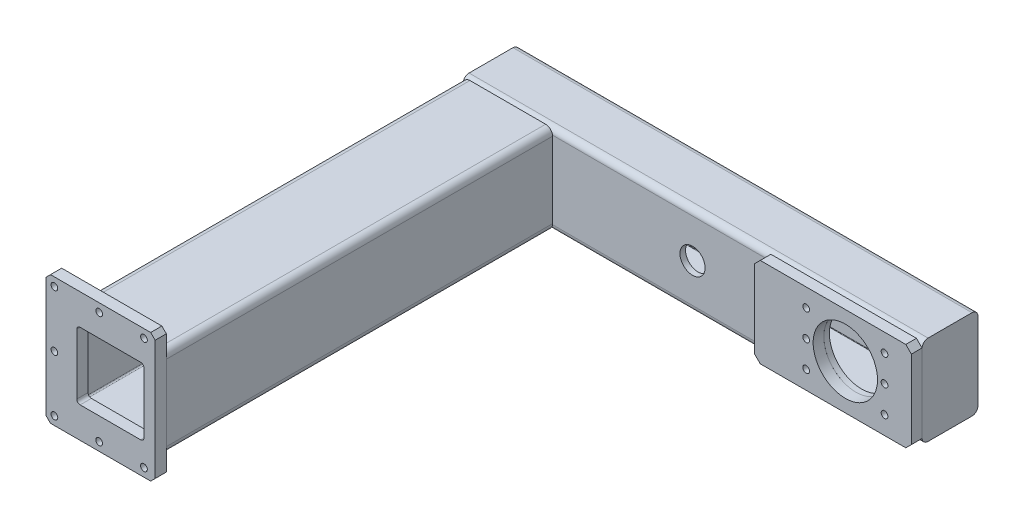
SolidWorks part; units mm, degrees
ref_plane "Front Plane" through (0, 0, 0) normal (0, 0, 1) x (1, 0, 0)
ref_plane "Top Plane" through (0, 0, 0) normal (0, 1, 0) x (1, 0, 0)
ref_plane "Right Plane" through (0, 0, 0) normal (1, 0, 0) x (0, 0, -1)
sketch "Sketch3" plane through (0, 0, 0) normal (0, 1, 0) x (1, 0, 0)
  line L0 (0, 0) -> (0, -740)
  line L1 (0, 0) -> (740, 0)
  dimension "D1" = 740
  dimension "D2" = 740
other "Structural Member1"
ref_plane "Plane1" through (0, 0, 0) normal (0, 0, 1) x (1, 0, 0)
sketch "Sketch1" plane through (0, 0, 0) normal (0, 0, 1) x (1, 0, 0)
  line L0 (-67.6073, -70) -> (67.6073, -70)
  line L1 (-70, -67.6073) -> (-70, 67.6073)
  line L2 (67.6073, 70) -> (-67.6073, 70)
  line L3 (70, 67.6073) -> (70, -67.6073)
  line L4 (-67.6073, -80) -> (67.6073, -80)
  line L5 (-80, -67.6073) -> (-80, 67.6073)
  line L6 (67.6073, 80) -> (-67.6073, 80)
  line L7 (80, 67.6073) -> (80, -67.6073)
  arc A0 (80, 67.6073) -> (67.6073, 80) centre (67.6073, 67.6073) ccw
  arc A1 (67.6073, -80) -> (80, -67.6073) centre (67.6073, -67.6073) ccw
  arc A2 (-80, -67.6073) -> (-67.6073, -80) centre (-67.6073, -67.6073) ccw
  arc A3 (-67.6073, 80) -> (-80, 67.6073) centre (-67.6073, 67.6073) ccw
  arc A4 (-67.6073, 70) -> (-70, 67.6073) centre (-67.6073, 67.6073) ccw
  arc A5 (70, 67.6073) -> (67.6073, 70) centre (67.6073, 67.6073) ccw
  arc A6 (67.6073, -70) -> (70, -67.6073) centre (67.6073, -67.6073) ccw
  arc A7 (-70, -67.6073) -> (-67.6073, -70) centre (-67.6073, -67.6073) ccw
  point P0 (-80, 0)
  point P1 (80, 0)
  point P2 (0, 80)
  point P3 (0, -80)
  point P4 (0, 0)
  point P5 (-80, -80)
  point P6 (80, -80)
  point P7 (80, 80)
  point P8 (-80, 80)
  point P33 (0, 0)
  dimension "Thickness" = 10
  dimension "V_leg" = 160
other "Structural Member2"
ref_plane "Plane2" through (0, 0, 0) normal (1, 0, 0) x (0, 0, -1)
sketch "Sketch11" plane through (0, 0, 0) normal (1, 0, 0) x (0, 0, -1)
  line L0 (-39.2141, -70) -> (39.2141, -70)
  line L1 (-40, -69.2141) -> (-40, 69.2141)
  line L2 (39.2141, 70) -> (-39.2141, 70)
  line L3 (40, 69.2141) -> (40, -69.2141)
  line L4 (-39.2141, -80) -> (39.2141, -80)
  line L5 (-50, -69.2141) -> (-50, 69.2141)
  line L6 (39.2141, 80) -> (-39.2141, 80)
  line L7 (50, 69.2141) -> (50, -69.2141)
  arc A0 (50, 69.2141) -> (39.2141, 80) centre (39.2141, 69.2141) ccw
  arc A1 (39.2141, -80) -> (50, -69.2141) centre (39.2141, -69.2141) ccw
  arc A2 (-50, -69.2141) -> (-39.2141, -80) centre (-39.2141, -69.2141) ccw
  arc A3 (-39.2141, 80) -> (-50, 69.2141) centre (-39.2141, 69.2141) ccw
  arc A4 (-39.2141, 70) -> (-40, 69.2141) centre (-39.2141, 69.2141) ccw
  arc A5 (40, 69.2141) -> (39.2141, 70) centre (39.2141, 69.2141) ccw
  arc A6 (39.2141, -70) -> (40, -69.2141) centre (39.2141, -69.2141) ccw
  arc A7 (-40, -69.2141) -> (-39.2141, -70) centre (-39.2141, -69.2141) ccw
  point P0 (-50, 0)
  point P1 (50, 0)
  point P2 (0, 80)
  point P3 (0, -80)
  point P4 (0, 0)
  point P5 (-50, -80)
  point P6 (50, -80)
  point P7 (50, 80)
  point P8 (-50, 80)
  point P33 (0, 0)
  dimension "D2" = 100
  dimension "Thickness" = 10
  dimension "V_leg" = 160
other "Trim/Extend1"
sketch "Sketch6" plane through (0, 0, 740) normal (0, 0, 1) x (1, 0, 0)
  line L0 (80, -67.6073) -> (80, 67.6073) construction
  line L1 (-115, 115) -> (80, 115)
  line L2 (-115, 115) -> (-115, -115)
  line L3 (-115, -115) -> (80, -115)
  line L4 (80, 115) -> (80, -115)
  line L5 (0, 0) -> (-106.3486, 0) construction
  dimension "D1" = 195
  dimension "D2" = 230
extrude "Boss-Extrude3" add sketch "Sketch6" along normal blind 20 separate body
sketch "Sketch7" plane through (0, 0, 50) normal (0, 0, 1) x (1, 0, 0)
  line L0 (740, 80) -> (-80, 80) construction
  line L1 (460, 80) -> (740, 80)
  line L2 (460, 80) -> (460, -80)
  line L3 (460, -80) -> (740, -80)
  line L4 (740, 80) -> (740, -80)
  dimension "D1" = 280
extrude "Boss-Extrude4" add sketch "Sketch7" along normal blind 19 separate body
sketch "Sketch8" plane through (0, 0, 50) normal (0, 0, 1) x (1, 0, 0)
  line L0 (740, 80) -> (-80, 80) construction
  line L1 (80, 80) -> (380, 80)
  line L2 (80, 80) -> (80, -80)
  line L3 (80, -80) -> (380, -80)
  line L4 (380, 80) -> (380, -80)
  line L5 (740, -80) -> (-80, -80) construction
  line L6 (80, 67.6073) -> (80, -67.6073) construction
  dimension "D1" = 300
sketch "Sketch12" plane through (0, 0, 69) normal (0, 0, 1) x (1, 0, 0)
  line L0 (740, 0) -> (622, 0) construction
  line L1 (740, -80) -> (740, 80) construction
  circle A0 centre (622, 0) radius 57.5
  dimension "D1" = 115
  dimension "D2" = 118
extrude "Cut-Extrude1" cut sketch "Sketch12" against normal blind 88
sketch "Sketch13" plane through (0, 0, 69) normal (0, 0, 1) x (1, 0, 0)
  line L0 (692, 47.5) -> (692, -47.5) construction
  line L1 (622, 0) -> (622, 100.2648) construction
  line L2 (622, 0) -> (692, 0) construction
  line L3 (552, 47.5) -> (552, -47.5) construction
  line L4 (552, 47.5) -> (715.5438, 47.5) construction
  circle A0 centre (692, 47.5) radius 6
  circle A1 centre (692, 0) radius 6
  circle A2 centre (692, -47.5) radius 6
  circle A3 centre (552, 47.5) radius 6
  circle A4 centre (552, 0) radius 6
  circle A5 centre (552, -47.5) radius 6
  dimension "D3" = 12
  dimension "D1" = 95
  dimension "D2" = 140
extrude "Cut-Extrude2" cut sketch "Sketch13" against normal blind 30
sketch "Sketch14" plane through (0, 0, -50) normal (0, 0, -1) x (-1, 0, 0)
  line L0 (0, 0) -> (-734.2171, 0) construction
  line L1 (-734.2171, 0) -> (-754.5804, 0) construction
  circle A0 centre (-622, 0) radius 41
  circle A1 centre (-330, 0) radius 22.5
  circle A2 centre (0, 0) radius 41
  dimension "D1" = 82
  dimension "D3" = 45
  dimension "D2" = 330
extrude "Cut-Extrude3" cut sketch "Sketch14" against normal through all
hole_wizard "M6 Tapped Hole1" positions "Sketch16" profile "Sketch15" tap size "M6" standard "Gb"
sketch "Sketch16" plane through (0, 0, -50) normal (0, 0, -1) x (-1, 0, 0)
  line L0 (-622, 0) -> (-622, -72.1924) construction
  circle A0 centre (-622, 0) radius 52.5 construction
  point P0 (-622, -52.5)
  dimension "D1" = 105
sketch "Sketch15" plane through (622, -52.5, -50) normal (1, 0, 0) x (0, 1, 0)
  line L0 (0, 0) -> (0, 16.5022)
  line L1 (0, 16.5022) -> (2.5, 15)
  line L2 (2.5, 15) -> (2.5, 0)
  line L5 (2.5, 0) -> (0, 0)
  line L10 (0, 16.5022) -> (-2.5, 15) construction
  line L11 (0, -6.35) -> (0, 107.95) construction
  dimension "螺纹孔钻头直径" = 5
  dimension "螺纹孔钻头深度" = 15
  dimension "导头角度" = 118
cosmetic thread "Cosmetic thread 1" parameters "D1"=10, "D2"=6
pattern_circular "CirPattern1" count 4 over 360 about axis through (622, 0, 0) along (0, 0, 1) of "M6 Tapped Hole1"
pattern_linear "LPattern1" count 2 spacing 622 along (-1, 0, 0) of "M6 Tapped Hole1", "CirPattern1"
sketch "Sketch17" plane through (0, 0, -50) normal (0, 0, -1) x (-1, 0, 0)
  line L0 (-622, 0) -> (237.989, 0) construction
  line L1 (-682, 50) -> (-725, 50)
  line L2 (-682, 50) -> (-682, -50)
  line L3 (-682, -50) -> (-725, -50)
  line L4 (-725, 50) -> (-725, -50)
  line L5 (-682, 50) -> (-725, -50) construction
  line L6 (-682, -50) -> (-725, 50) construction
  line L7 (-740, -69.2141) -> (-740, 69.2141) construction
  line L8 (-65, 50) -> (-290, 50)
  line L9 (-65, 50) -> (-65, -50)
  line L10 (-65, -50) -> (-290, -50)
  line L11 (-290, 50) -> (-290, -50)
  line L12 (-65, 50) -> (-290, -50) construction
  line L13 (-65, -50) -> (-290, 50) construction
  line L14 (-562, 50) -> (-370, 50)
  line L15 (-562, 50) -> (-562, -50)
  line L16 (-562, -50) -> (-370, -50)
  line L17 (-370, 50) -> (-370, -50)
  line L18 (-562, 50) -> (-370, -50) construction
  line L19 (-562, -50) -> (-370, 50) construction
  point P0 (-703.5, 0)
  point P9 (-177.5, 0)
  point P14 (-466, 0)
  dimension "D1" = 15
  dimension "D2" = 43
  dimension "D3" = 100
  dimension "D4" = 192
  dimension "D5" = 225
  dimension "D6" = 392
  dimension "D7" = 120
extrude "Cut-Extrude4" cut sketch "Sketch17" against normal blind 10
fillet "Fillet1" radius 6 12 edges at (682, 50, -45) (370, 50, -45) (290, 50, -45) (562, 50, -45) (725, 50, -45) (290, -50, -45) (562, -50, -45) (725, -50, -45) (682, -50, -45) (370, -50, -45) (65, 50, -45) (65, -50, -45)
hole_wizard "M4 Tapped Hole1" positions "Sketch19" profile "Sketch18" tap size "M4" standard "Gb"
sketch "Sketch19" plane through (0, 0, -50) normal (0, 0, -1) x (-1, 0, 0)
  line L0 (-330, 0) -> (-359.8714, -29.8714) construction
  line L2 (-330, 0) -> (-330, -35.2441) construction
  circle A0 centre (-330, 0) radius 36.0624
  point P0 (-355.5, -25.5)
  dimension "D1" = 51
  dimension "D2" = 45
sketch "Sketch18" plane through (355.5, -25.5, -50) normal (1, 0, 0) x (0, 1, 0)
  line L0 (0, 0) -> (0, 11.0914)
  line L1 (0, 11.0914) -> (1.65, 10.1)
  line L2 (1.65, 10.1) -> (1.65, 0)
  line L5 (1.65, 0) -> (0, 0)
  line L10 (0, 11.0914) -> (-1.65, 10.1) construction
  line L11 (0, -6.35) -> (0, 107.95) construction
  dimension "螺纹孔钻头直径" = 3.3
  dimension "螺纹孔钻头深度" = 10.1
  dimension "导头角度" = 118
cosmetic thread "Cosmetic thread 2" parameters "D1"=8, "D2"=4
pattern_circular "CirPattern2" count 4 over 360 about axis through (330, 0, 0) along (0, 0, 1) of "M4 Tapped Hole1"
sketch "Sketch20" plane through (0, 0, 40) normal (0, 0, -1) x (-1, 0, 0)
  circle A0 centre (0, 0) radius 57.5
  dimension "D1" = 115
sketch "Sketch21" plane through (0, 0, 40) normal (0, 0, -1) x (-1, 0, 0)
  line L1 (-57.5, 57.5) -> (57.5, 57.5)
  line L2 (-57.5, 57.5) -> (-57.5, -57.5)
  line L3 (-57.5, -57.5) -> (57.5, -57.5)
  line L4 (57.5, 57.5) -> (57.5, -57.5)
  line L5 (-57.5, 57.5) -> (57.5, -57.5) construction
  line L6 (-57.5, -57.5) -> (57.5, 57.5) construction
  point P0 (0, 0)
  dimension "D1" = 115
extrude "Cut-Extrude6" cut sketch "Sketch21" against normal blind 51
fillet "Fillet2" radius 6 4 edges at (57.5, 57.5, 45) (-57.5, 57.5, 45) (57.5, -57.5, 45) (-57.5, -57.5, 45)
sketch "Sketch22" plane through (-80, 0, 0) normal (-1, 0, 0) x (0, 0, 1)
  line L1 (41.181, -71.5885) -> (-41.181, -71.5885)
  line L2 (41.181, -71.5885) -> (41.181, 71.5885)
  line L3 (41.181, 71.5885) -> (-41.181, 71.5885)
  line L4 (-41.181, -71.5885) -> (-41.181, 71.5885)
  line L5 (41.181, -71.5885) -> (-41.181, 71.5885) construction
  line L6 (41.181, 71.5885) -> (-41.181, -71.5885) construction
  point P0 (0, 0)
extrude "Boss-Extrude9" add sketch "Sketch22" against normal blind 5
sketch "Sketch23" plane through (740, 0, 0) normal (1, 0, 0) x (0, 0, -1)
  line L1 (-40.8602, 71.7017) -> (40.8602, 71.7017)
  line L2 (-40.8602, 71.7017) -> (-40.8602, -71.7017)
  line L3 (-40.8602, -71.7017) -> (40.8602, -71.7017)
  line L4 (40.8602, 71.7017) -> (40.8602, -71.7017)
  line L5 (-40.8602, 71.7017) -> (40.8602, -71.7017) construction
  line L6 (-40.8602, -71.7017) -> (40.8602, 71.7017) construction
  point P0 (0, 0)
extrude "Boss-Extrude10" add sketch "Sketch23" against normal blind 5
hole_wizard "M4 Tapped Hole2" positions "Sketch25" profile "Sketch24" tap size "M4" standard "Gb"
sketch "Sketch25" plane through (0, 0, -50) normal (0, 0, -1) x (-1, 0, 0)
  line L0 (-55, -45) -> (-794.005, -45) construction
  line L2 (-55, 45) -> (-804.2358, 45) construction
  line L4 (80, 69.2141) -> (80, -69.2141) construction
  line L5 (-330, 0) -> (-330, -115.362) construction
  line L7 (-622, 0) -> (-622, -115.362) construction
  line L9 (-622, 0) -> (-800.4528, 0) construction
  line L10 (-55, -45) -> (-55, 96.3703) construction
  line L12 (-677, -45) -> (-677, 90.0804) construction
  line L14 (-740, -69.2141) -> (-740, 69.2141) construction
  line L15 (-730, -25) -> (-730, 24.414) construction
  point P0 (-55, -45)
  point P2 (-55, 45)
  point P4 (-330, 45)
  point P6 (-330, -45)
  point P8 (-567, -45)
  point P10 (-567, 45)
  point P12 (-677, 45)
  point P14 (-677, -45)
  point P16 (-730, -25)
  point P18 (-730, 25)
  dimension "D1" = 90
  dimension "D2" = 135
  dimension "D3" = 237
  dimension "D4" = 50
  dimension "D5" = 10
sketch "Sketch24" plane through (55, -45, -50) normal (1, 0, 0) x (0, 1, 0)
  line L0 (0, 0) -> (0, 11.0914)
  line L1 (0, 11.0914) -> (1.65, 10.1)
  line L2 (1.65, 10.1) -> (1.65, 0)
  line L5 (1.65, 0) -> (0, 0)
  line L10 (0, 11.0914) -> (-1.65, 10.1) construction
  line L11 (0, -6.35) -> (0, 107.95) construction
  dimension "螺纹孔钻头直径" = 3.3
  dimension "螺纹孔钻头深度" = 10.1
  dimension "导头角度" = 118
cosmetic thread "Cosmetic thread 3" parameters "D1"=8, "D2"=4
cosmetic thread "Cosmetic thread 4" parameters "D1"=8, "D2"=4
cosmetic thread "Cosmetic thread 5" parameters "D1"=8, "D2"=4
cosmetic thread "Cosmetic thread 6" parameters "D1"=8, "D2"=4
cosmetic thread "Cosmetic thread 7" parameters "D1"=8, "D2"=4
cosmetic thread "Cosmetic thread 8" parameters "D1"=8, "D2"=4
cosmetic thread "Cosmetic thread 9" parameters "D1"=8, "D2"=4
cosmetic thread "Cosmetic thread 10" parameters "D1"=8, "D2"=4
cosmetic thread "Cosmetic thread 11" parameters "D1"=8, "D2"=4
cosmetic thread "Cosmetic thread 12" parameters "D1"=8, "D2"=4
hole_wizard "Ø12.0 (12) Diameter Hole1" positions "Sketch27" profile "Sketch26" hole size "Ø12.0" standard "Gb" end condition through all
sketch "Sketch27" plane through (0, 0, 760) normal (0, 0, 1) x (1, 0, 0)
  line L0 (0, 0) -> (-175.4043, 0) construction
  line L1 (-100, 100) -> (-100, -100) construction
  line L3 (-100, 100) -> (60, 100) construction
  line L5 (-100, -100) -> (60, -100) construction
  line L7 (-115, 115) -> (-115, -115) construction
  line L8 (-115, -115) -> (80, -115) construction
  line L9 (80, 115) -> (-115, 115) construction
  line L10 (80, -115) -> (80, 115) construction
  line L11 (-20, -100) -> (-20, 155.6721) construction
  line L13 (60, -100) -> (60, 152.6721) construction
  point P0 (-100, -100)
  point P2 (-20, -100)
  point P4 (60, -100)
  point P6 (-100, 100)
  point P8 (-20, 100)
  point P10 (60, 100)
  point P17 (-100, 0)
  dimension "D1" = 15
  dimension "D2" = 15
  dimension "D3" = 15
  dimension "D5" = 20
sketch "Sketch26" plane through (-100, -100, 760) normal (1, 0, 0) x (0, -1, 0)
  line L0 (0, 0) -> (0, 810)
  line L1 (0, 810) -> (6, 810)
  line L2 (6, 810) -> (6, 0)
  line L5 (6, 0) -> (0, 0)
  line L11 (0, -6.35) -> (0, 107.95) construction
  dimension "通孔孔直径" = 12
  dimension "通孔孔深度" = 810
chamfer "Chamfer1" distance 8 angle 45 4 edges at (80, -115, 750) (-115, -115, 750) (80, 115, 750) (-115, 115, 750)
chamfer "Chamfer2" distance 10 angle 45 4 edges at (460, -80, 59.5) (460, 80, 59.5) (740, -80, 59.5) (740, 80, 59.5)
sketch "Sketch28" plane through (0, 0, 760) normal (0, 0, 1) x (1, 0, 0)
  line L0 (0, 0) -> (112.3575, 0) construction
  line L1 (-60, 60) -> (60, 60)
  line L2 (-60, 60) -> (-60, -60)
  line L3 (-60, -60) -> (60, -60)
  line L4 (60, 60) -> (60, -60)
  line L5 (80, -107) -> (80, 107) construction
  dimension "D1" = 120
  dimension "D2" = 20
  dimension "D3" = 120
extrude "Cut-Extrude7" cut sketch "Sketch28" against normal blind 65
fillet "Fillet3" radius 6 4 edges at (60, 60, 750) (60, -60, 750) (-60, -60, 750) (-60, 60, 750)
